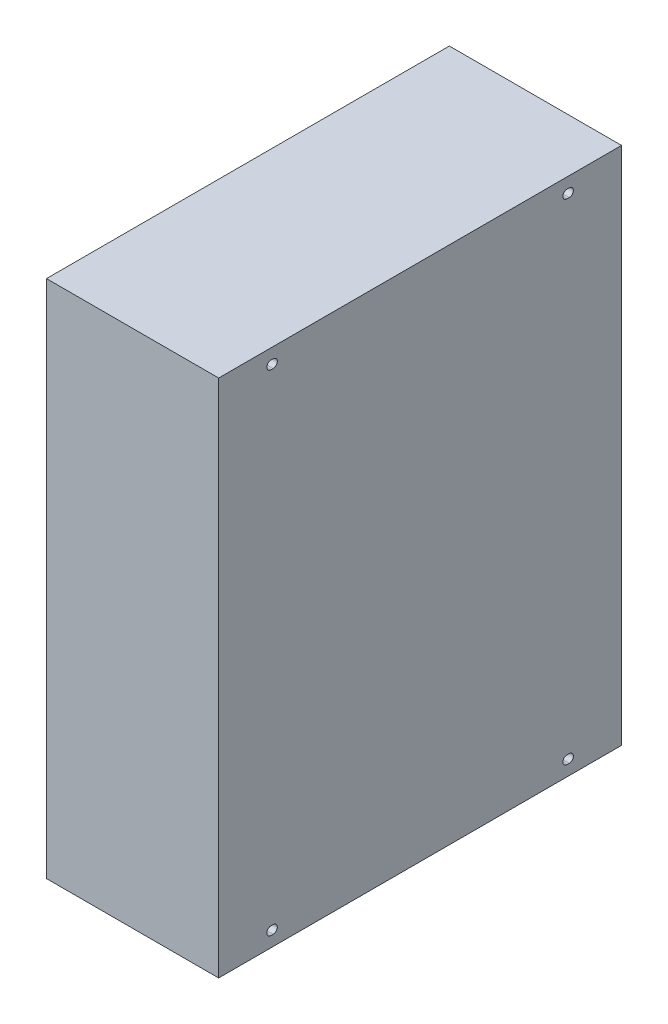
from build123d import *

# Parameters (mm, degrees)
SKETCH_1_W          = 575.6
SKETCH_1_H          = 742.4
EXTRUDE_1_DEPTH     = 123
CUT_EXTRUDE_1_DEPTH = 531.220972803


with BuildPart() as part:
    # 草图1 → 凸台-拉伸1 (new, symmetric)
    with BuildSketch(Plane(origin=(0, 0, 0), x_dir=(0, 0, -1), z_dir=(1, 0, 0))):
        Rectangle(SKETCH_1_W, SKETCH_1_H)
    extrude(amount=EXTRUDE_1_DEPTH, both=True)

    # 草图2 → 切除-拉伸1 (cut, through all)
    with BuildSketch(Plane(origin=(123, 0, 0), x_dir=(0, 0, -1), z_dir=(1, 0, 0))):
        with BuildLine():
            Line((-213, 356), (-210, 356))
            ThreePointArc((-210, 356), (-204, 350), (-210, 344))
            Line((-210, 344), (-213, 344))
            ThreePointArc((-213, 344), (-219, 350), (-213, 356))
        make_face()
        with BuildLine():
            Line((210, 356), (213, 356))
            ThreePointArc((213, 356), (219, 350), (213, 344))
            Line((213, 344), (210, 344))
            ThreePointArc((210, 344), (204, 350), (210, 356))
        make_face()
        with BuildLine():
            Line((210, -344), (213, -344))
            ThreePointArc((213, -344), (219, -350), (213, -356))
            Line((213, -356), (210, -356))
            ThreePointArc((210, -356), (204, -350), (210, -344))
        make_face()
        with BuildLine():
            Line((-213, -344), (-210, -344))
            ThreePointArc((-210, -344), (-204, -350), (-210, -356))
            Line((-210, -356), (-213, -356))
            ThreePointArc((-213, -356), (-219, -350), (-213, -344))
        make_face()
    extrude(amount=-CUT_EXTRUDE_1_DEPTH, mode=Mode.SUBTRACT)


solid = part.part
